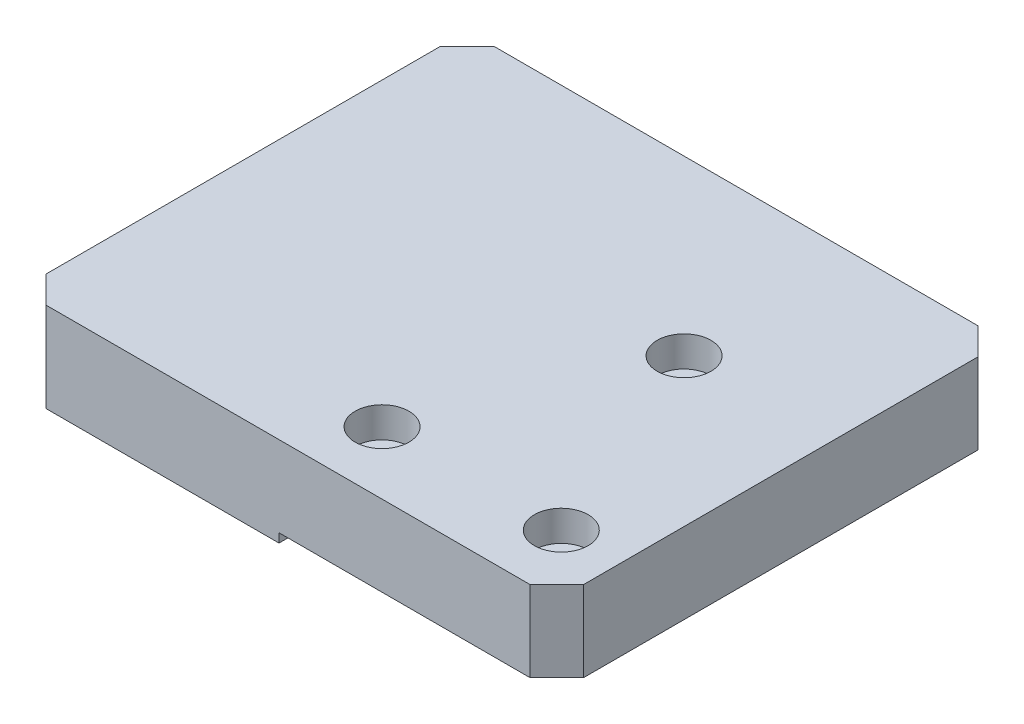
from build123d import *

# Parameters (mm, degrees)
SKETCH_1_W                = 60
SKETCH_1_H                = 50
EXTRUDE_1_DEPTH           = 10
SKETCH_5_W                = 31
SKETCH_5_H                = 50
CUT_EXTRUDE_1_DEPTH       = 1
CHAMFER_2_SIZE            = 3
HOLE_WIZARD_M5_1_D        = 4.2
HOLE_WIZARD_M5_1_DEPTH    = 12.4
HOLE_WIZARD_M5_1_TIP      = 1.2618073
HOLE_WIZARD_3_D           = 3.4
HOLE_WIZARD_3_DEPTH       = 12.4
HOLE_WIZARD_3_CBORE_D     = 6
HOLE_WIZARD_3_CBORE_DEPTH = 3.4
HOLE_WIZARD_3_TIP         = 1.021463052
MM_3_D                    = 4
MM_3_DEPTH                = 12.4
MM_3_TIP                  = 1.201721238


with BuildPart() as part:
    # 草图1 → 凸台-拉伸1 (new body)
    with BuildSketch(Plane(origin=(0, 0, 0), x_dir=(1, 0, 0), z_dir=(0, 1, 0))):
        Rectangle(SKETCH_1_W, SKETCH_1_H)
    extrude(amount=EXTRUDE_1_DEPTH)

    # 草图5 → 切除-拉伸1 (cut)
    with BuildSketch(Plane.XZ):
        with Locations((14.5, 0)):
            Rectangle(SKETCH_5_W, SKETCH_5_H)
    extrude(amount=-CUT_EXTRUDE_1_DEPTH, mode=Mode.SUBTRACT)

    # 倒角2
    chamfer_2_edges = [part.edges().sort_by_distance(p)[0] for p in [
        (30, 5.5, 25),
        (-30, 5, 25),
        (-30, 5, -25),
        (30, 5.5, -25),
    ]]
    chamfer(chamfer_2_edges, length=CHAMFER_2_SIZE)

    # M5 螺纹孔1
    with Locations(Plane.ZY.offset(30)):
        with Locations((17, 5), (-17, 4.974257895), (0, 4.974257895)):
            Hole(HOLE_WIZARD_M5_1_D / 2, depth=HOLE_WIZARD_M5_1_DEPTH)
            with Locations((0, 0, -(HOLE_WIZARD_M5_1_DEPTH + HOLE_WIZARD_M5_1_TIP / 2))):  # 118° drill point
                Cone(0, HOLE_WIZARD_M5_1_D / 2, HOLE_WIZARD_M5_1_TIP, mode=Mode.SUBTRACT)

    # 打孔尺寸(%根据)内六角圆柱头螺钉的类型3
    with Locations(Plane(origin=(0, 10, 0), x_dir=(1, 0, 0), z_dir=(0, 1, 0))):
        with Locations((23.5, -18), (3.5, -18), (13.5, 5.7)):
            CounterBoreHole(HOLE_WIZARD_3_D / 2, HOLE_WIZARD_3_CBORE_D / 2, HOLE_WIZARD_3_CBORE_DEPTH, depth=HOLE_WIZARD_3_DEPTH)
            with Locations((0, 0, -(HOLE_WIZARD_3_DEPTH + HOLE_WIZARD_3_TIP / 2))):  # 118° drill point
                Cone(0, HOLE_WIZARD_3_D / 2, HOLE_WIZARD_3_TIP, mode=Mode.SUBTRACT)

    # 大小mm 暗销孔3
    with Locations(Plane.ZY.offset(30)):
        with Locations((9, 5), (-9, 5)):
            Hole(MM_3_D / 2, depth=MM_3_DEPTH)
            with Locations((0, 0, -(MM_3_DEPTH + MM_3_TIP / 2))):  # 118° drill point
                Cone(0, MM_3_D / 2, MM_3_TIP, mode=Mode.SUBTRACT)


solid = part.part
